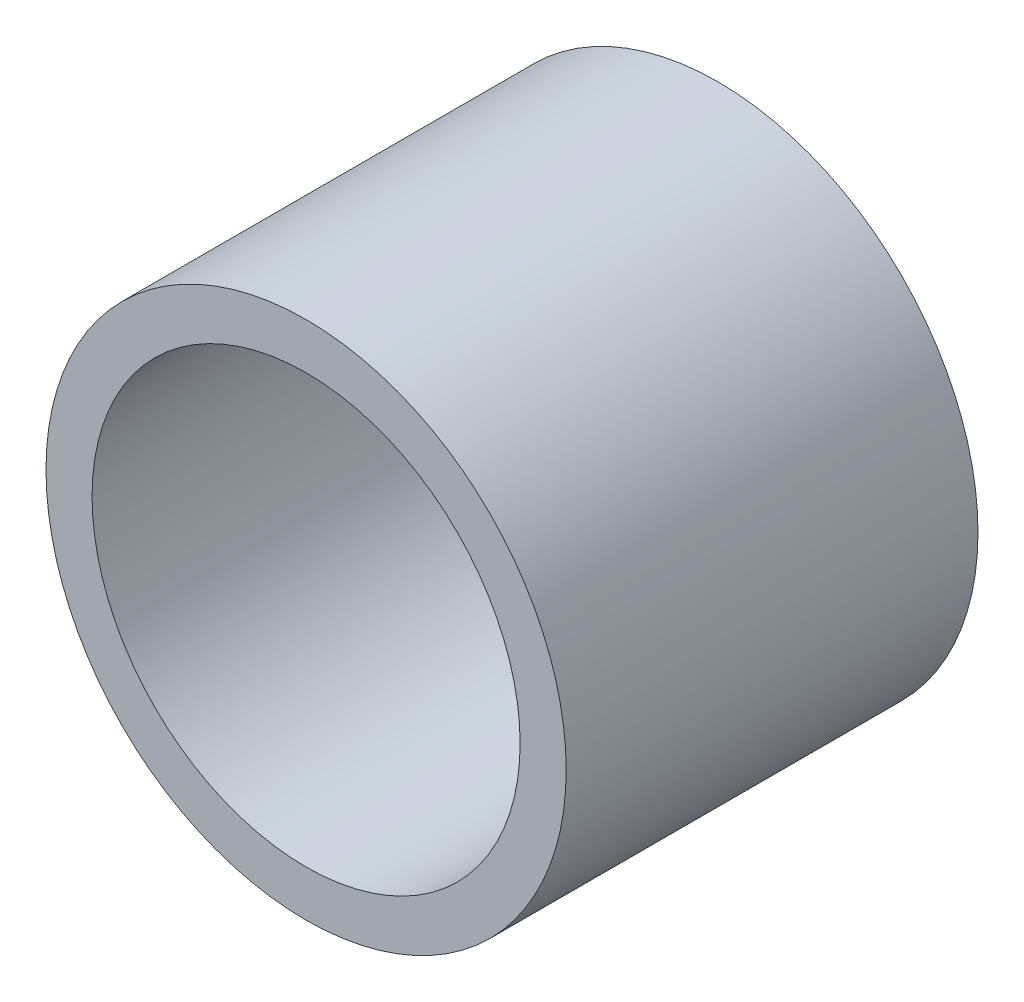
from build123d import *

# Parameters (mm, degrees)
SKETCH1_R           = 24
SKETCH1_R_2         = 19.75
BOSS_EXTRUDE1_DEPTH = 19


with BuildPart() as part:
    # Sketch1 → Boss-Extrude1 (new, symmetric)
    with BuildSketch(Plane.XY):
        Circle(SKETCH1_R)
        Circle(SKETCH1_R_2, mode=Mode.SUBTRACT)
    extrude(amount=BOSS_EXTRUDE1_DEPTH, both=True)


solid = part.part
